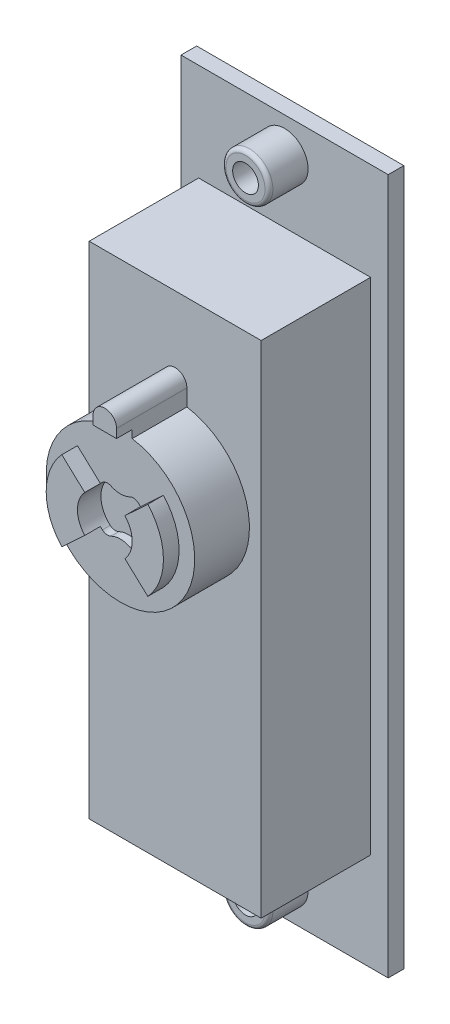
from build123d import *

# Parameters (mm, degrees)
SKETCH1_W             = 26.5
SKETCH1_H             = 89
BOSS_EXTRUDE1_DEPTH   = 3
SKETCH2_W             = 22
SKETCH2_H             = 64
BOSS_EXTRUDE2_DEPTH   = 14
SKETCH3_R             = 3
BOSS_EXTRUDE3_DEPTH   = 5
M4_TAPPED_HOLE1_D     = 3.3
M4_TAPPED_HOLE1_DEPTH = 5
M4_TAPPED_HOLE1_TIP   = 0.991420021
CHAMFER1_SIZE         = 3
CHAMFER1_SIZE2        = 1
SKETCH6_R             = 9.5
BOSS_EXTRUDE4_DEPTH   = 7
BOSS_EXTRUDE5_DEPTH   = 9
CUT_EXTRUDE1_START    = -2
CUT_EXTRUDE1_DEPTH    = 2
SKETCH9_R             = 7.5
BOSS_EXTRUDE6_DEPTH   = 2
CUT_EXTRUDE5_DEPTH    = 3
CUT_EXTRUDE6_DEPTH    = 2
SKETCH14_R            = 6.5
BOSS_EXTRUDE7_DEPTH   = 3
CUT_EXTRUDE7_START    = -2.5
CUT_EXTRUDE7_DEPTH    = 2.5
FILLET1_R             = 1
BOSS_EXTRUDE8_DEPTH   = 3
FILLET2_R             = 1
FILLET3_R             = 0.5


with BuildPart() as part:
    # Sketch1 → Boss-Extrude1 (new body)
    with BuildSketch(Plane.XY):
        Rectangle(SKETCH1_W, SKETCH1_H)
    extrude(amount=BOSS_EXTRUDE1_DEPTH)

    # Sketch2 → Boss-Extrude2 (add)
    with BuildSketch(Plane.XY.offset(3)):
        Rectangle(SKETCH2_W, SKETCH2_H)
    extrude(amount=BOSS_EXTRUDE2_DEPTH)

    # Sketch3 → Boss-Extrude3 (add)
    with BuildSketch(Plane.XY.offset(3)):
        with Locations(Location((0, 40, 0), (0, 0, 180))):
            Circle(SKETCH3_R)
        with Locations(Location((0, -40, 0), (0, 0, 180))):
            Circle(SKETCH3_R)
    extrude(amount=BOSS_EXTRUDE3_DEPTH)

    # M4 Tapped Hole1
    with Locations(Plane.XY.offset(8)):
        with Locations((0, 40), (0, -40)):
            Hole(M4_TAPPED_HOLE1_D / 2, depth=M4_TAPPED_HOLE1_DEPTH)
            with Locations((0, 0, -(M4_TAPPED_HOLE1_DEPTH + M4_TAPPED_HOLE1_TIP / 2))):  # 118° drill point
                Cone(0, M4_TAPPED_HOLE1_D / 2, M4_TAPPED_HOLE1_TIP, mode=Mode.SUBTRACT)

    # Chamfer1
    chamfer1_edges = [part.edges().sort_by_distance(p)[0] for p in [
        (0, -44.5, 0),
        (-13.25, 0, 0),
        (0, 44.5, 0),
        (13.25, 0, 0),
    ]]
    chamfer1_side = [part.faces().sort_by_distance(p)[0] for p in [
        (0, 0, 0),
    ]]
    chamfer(chamfer1_edges, length=CHAMFER1_SIZE, length2=CHAMFER1_SIZE2, reference=chamfer1_side[0])

    # Sketch6 → Boss-Extrude4 (add)
    with BuildSketch(Plane.XY.offset(17)):
        with Locations(Location((0, 10.5, 0), (0, 0, 180))):
            Circle(SKETCH6_R)
    extrude(amount=BOSS_EXTRUDE4_DEPTH)

    # Sketch7 → Boss-Extrude5 (add)
    with BuildSketch(Plane.XY.offset(17)):
        with BuildLine():
            Line((-1.5, 19.88083152), (-1.5, 22))
            ThreePointArc((-1.5, 22), (0, 23.5), (1.5, 22))
            Line((1.5, 22), (1.5, 19.88083152))
            ThreePointArc((1.5, 19.88083152), (0, 20), (-1.5, 19.88083152))
        make_face()
    extrude(amount=BOSS_EXTRUDE5_DEPTH)

    # Sketch8 → Cut-Extrude1 (cut)
    with BuildSketch(Plane.XY.offset(26).offset(CUT_EXTRUDE1_START)):
        with BuildLine():
            Line((1.5, 20.88083152), (-1.5, 20.88083152))
            Line((-1.5, 20.88083152), (-1.5, 19.88083152))
            ThreePointArc((-1.5, 19.88083152), (0, 20), (1.5, 19.88083152))
            Line((1.5, 19.88083152), (1.5, 20.88083152))
        make_face()
    extrude(amount=CUT_EXTRUDE1_DEPTH, mode=Mode.SUBTRACT)

    # Sketch9 → Boss-Extrude6 (add)
    with BuildSketch(Plane.XY.offset(24)):
        with Locations((0, 10.5)):
            Circle(SKETCH9_R)
    extrude(amount=BOSS_EXTRUDE6_DEPTH)

    # Sketch12 → Cut-Extrude5 (cut)
    with BuildSketch(Plane.XY.offset(26)):
        with BuildLine():
            ThreePointArc((-2.305548862, 13.133333333), (-3.5, 10.5), (-2.305548862, 7.866666667))
            ThreePointArc((-2.305548862, 7.866666667), (-1.778671788, 7.627778095), (-1.207668452, 7.720634921))
            ThreePointArc((-1.207668452, 7.720634921), (0, 8), (1.207668452, 7.720634921))
            ThreePointArc((1.207668452, 7.720634921), (1.778671788, 7.627778095), (2.305548862, 7.866666667))
            ThreePointArc((2.305548862, 7.866666667), (3.5, 10.5), (2.305548862, 13.133333333))
            ThreePointArc((2.305548862, 13.133333333), (1.778671788, 13.372221905), (1.207668452, 13.279365079))
            ThreePointArc((1.207668452, 13.279365079), (0, 13), (-1.207668452, 13.279365079))
            ThreePointArc((-1.207668452, 13.279365079), (-1.778671788, 13.372221905), (-2.305548862, 13.133333333))
        make_face()
    extrude(amount=-CUT_EXTRUDE5_DEPTH, mode=Mode.SUBTRACT)

    # Sketch13 → Cut-Extrude6 (cut)
    with BuildSketch(Plane.XY.offset(26)):
        with BuildLine():
            Line((2.566666667, 12.87954244), (5.5, 15.599019514))
            ThreePointArc((5.5, 15.599019514), (0, 18), (-5.5, 15.599019514))
            Line((-5.5, 15.599019514), (-2.566666667, 12.87954244))
            ThreePointArc((-2.566666667, 12.87954244), (-2.439410481, 13.009835952), (-2.305548862, 13.133333333))
            ThreePointArc((-2.305548862, 13.133333333), (-1.778671788, 13.372221905), (-1.207668452, 13.279365079))
            ThreePointArc((-1.207668452, 13.279365079), (0, 13), (1.207668452, 13.279365079))
            ThreePointArc((1.207668452, 13.279365079), (1.778671788, 13.372221905), (2.305548862, 13.133333333))
            ThreePointArc((2.305548862, 13.133333333), (2.439410481, 13.009835952), (2.566666667, 12.87954244))
        make_face()
        with BuildLine():
            Line((-2.566666667, 8.12045756), (-5.5, 5.400980486))
            ThreePointArc((-5.5, 5.400980486), (0, 3), (5.5, 5.400980486))
            Line((5.5, 5.400980486), (2.566666667, 8.12045756))
            ThreePointArc((2.566666667, 8.12045756), (2.439410481, 7.990164048), (2.305548862, 7.866666667))
            ThreePointArc((2.305548862, 7.866666667), (1.778671788, 7.627778095), (1.207668452, 7.720634921))
            ThreePointArc((1.207668452, 7.720634921), (0, 8), (-1.207668452, 7.720634921))
            ThreePointArc((-1.207668452, 7.720634921), (-1.778671788, 7.627778095), (-2.305548862, 7.866666667))
            ThreePointArc((-2.305548862, 7.866666667), (-2.439410481, 7.990164048), (-2.566666667, 8.12045756))
        make_face()
    extrude(amount=-CUT_EXTRUDE6_DEPTH, mode=Mode.SUBTRACT)

    # Sketch14 → Boss-Extrude7 (add)
    with BuildSketch(Plane(origin=(0, 0, 0), x_dir=(-1, 0, 0), z_dir=(0, 0, -1))):
        with Locations((0, -15.5)):
            Circle(SKETCH14_R)
    extrude(amount=BOSS_EXTRUDE7_DEPTH)

    # Sketch15 → Cut-Extrude7 (cut)
    with BuildSketch(Plane(origin=(0, 0, -3), x_dir=(-1, 0, 0), z_dir=(0, 0, -1)).offset(CUT_EXTRUDE7_START)):
        with BuildLine():
            Line((1.5, -17), (6.32455532, -17))
            ThreePointArc((6.32455532, -17), (6.5, -15.5), (6.32455532, -14))
            Line((6.32455532, -14), (1.5, -14))
            Line((1.5, -14), (1.5, -17))
        make_face()
        with BuildLine():
            Line((-1.5, -14), (-6.32455532, -14))
            ThreePointArc((-6.32455532, -14), (-6.5, -15.5), (-6.32455532, -17))
            Line((-6.32455532, -17), (-1.5, -17))
            Line((-1.5, -17), (-1.5, -14))
        make_face()
    extrude(amount=CUT_EXTRUDE7_DEPTH, mode=Mode.SUBTRACT)

    # Fillet1
    fillet1_edges = [part.edges().sort_by_distance(p)[0] for p in [
        (0, -9, -3),
        (-3.91227766, -14, -3),
        (-1.5, -15.5, -3),
        (-3.91227766, -17, -3),
        (0, -22, -3),
        (1.5, -15.5, -3),
        (3.91227766, -14, -3),
        (3.91227766, -17, -3),
    ]]
    fillet(fillet1_edges, radius=FILLET1_R)

    # Sketch16 → Boss-Extrude8 (add)
    with BuildSketch(Plane(origin=(0, 0, 0), x_dir=(-1, 0, 0), z_dir=(0, 0, -1))):
        with BuildLine():
            Line((-2.822662236, 32.659271568), (-8.634182974, 16.516158405))
            ThreePointArc((-8.634182974, 16.516158405), (-8.811520739, 15.5), (-8.634182974, 14.483841595))
            Line((-8.634182974, 14.483841595), (-2.822662236, -1.659271568))
            ThreePointArc((-2.822662236, -1.659271568), (0, -3.643113163), (2.822662236, -1.659271568))
            Line((2.822662236, -1.659271568), (8.634182974, 14.483841595))
            ThreePointArc((8.634182974, 14.483841595), (8.811520739, 15.5), (8.634182974, 16.516158405))
            Line((8.634182974, 16.516158405), (2.822662236, 32.659271568))
            ThreePointArc((2.822662236, 32.659271568), (0, 34.643113163), (-2.822662236, 32.659271568))
        make_face()
    extrude(amount=BOSS_EXTRUDE8_DEPTH)

    # Fillet2
    fillet2_edges = [part.edges().sort_by_distance(p)[0] for p in [
        (0, -3.643113163, -3),
        (-5.728422605, 6.412285014, -3),
        (-8.811520739, 15.5, -3),
        (-5.728422605, 24.587714986, -3),
        (0, 34.643113163, -3),
        (5.728422605, 24.587714986, -3),
        (8.811520739, 15.5, -3),
        (5.728422605, 6.412285014, -3),
    ]]
    fillet(fillet2_edges, radius=FILLET2_R)

    # Fillet3
    fillet3_edges = [part.edges().sort_by_distance(p)[0] for p in [
        (3, 40, 8),
        (3, -40, 8),
    ]]
    fillet(fillet3_edges, radius=FILLET3_R)


solid = part.part
